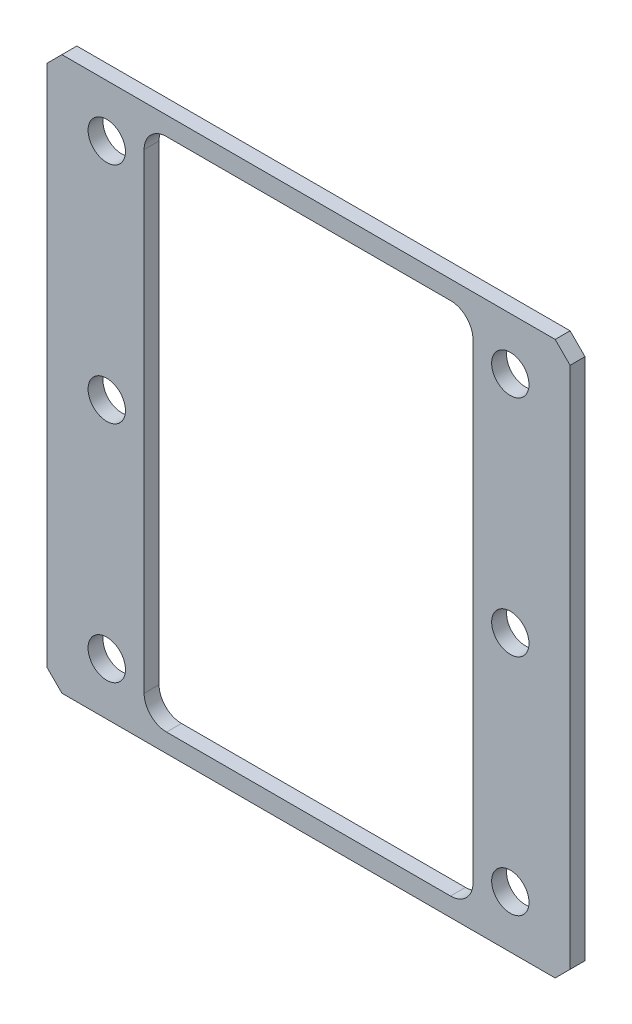
SolidWorks part; units mm, degrees
material "Q235-A"
ref_plane "Front Plane" through (0, 0, 0) normal (0, 0, 1) x (1, 0, 0)
ref_plane "Top Plane" through (0, 0, 0) normal (0, 1, 0) x (1, 0, 0)
ref_plane "Right Plane" through (0, 0, 0) normal (1, 0, 0) x (0, 0, -1)
sketch "Sketch1" plane through (0, 0, 0) normal (0, 0, 1) x (1, 0, 0)
  line L0 (-27, 0) -> (27, 0) construction
  line L1 (-35, -37) -> (35, -37)
  line L2 (-35, -37) -> (-35, 37)
  line L3 (-35, 37) -> (35, 37)
  line L4 (35, -37) -> (35, 37)
  line L5 (-35, -37) -> (35, 37) construction
  line L6 (-35, 37) -> (35, -37) construction
  line L7 (-19, -34.5) -> (19, -34.5)
  line L8 (-22, -31.5) -> (-22, 31.5)
  line L9 (-19, 34.5) -> (19, 34.5)
  line L10 (22, -31.5) -> (22, 31.5)
  line L11 (-22, -34.5) -> (22, 34.5) construction
  line L12 (-22, 34.5) -> (22, -34.5) construction
  line L13 (-27, -30) -> (27, -30) construction
  line L14 (-27, -30) -> (-27, 30) construction
  line L15 (-27, 30) -> (27, 30) construction
  line L16 (27, -30) -> (27, 30) construction
  line L17 (-27, -30) -> (27, 30) construction
  line L18 (-27, 30) -> (27, -30) construction
  arc A0 (19, 34.5) -> (22, 31.5) centre (19, 31.5) cw
  arc A1 (22, -31.5) -> (19, -34.5) centre (19, -31.5) cw
  arc A2 (-19, -34.5) -> (-22, -31.5) centre (-19, -31.5) cw
  arc A3 (-22, 31.5) -> (-19, 34.5) centre (-19, 31.5) cw
  circle A4 centre (-27, 30) radius 2.5
  circle A5 centre (-27, 0) radius 2.5
  circle A6 centre (-27, -30) radius 2.5
  circle A7 centre (27, -30) radius 2.5
  circle A8 centre (27, 0) radius 2.5
  circle A9 centre (27, 30) radius 2.5
  point P0 (0, 0)
  point P6 (0, 0)
  point P23 (0, 0)
  dimension "D5" = 3
  dimension "D1" = 74
  dimension "D2" = 70
  dimension "D3" = 44
  dimension "D4" = 69
  dimension "D6" = 60
  dimension "D7" = 54
extrude "Boss-Extrude1" add sketch "Sketch1" along normal blind 2
chamfer "Chamfer1" distance 2 angle 45 4 edges at (35, -37, 1) (35, 37, 1) (-35, -37, 1) (-35, 37, 1)
